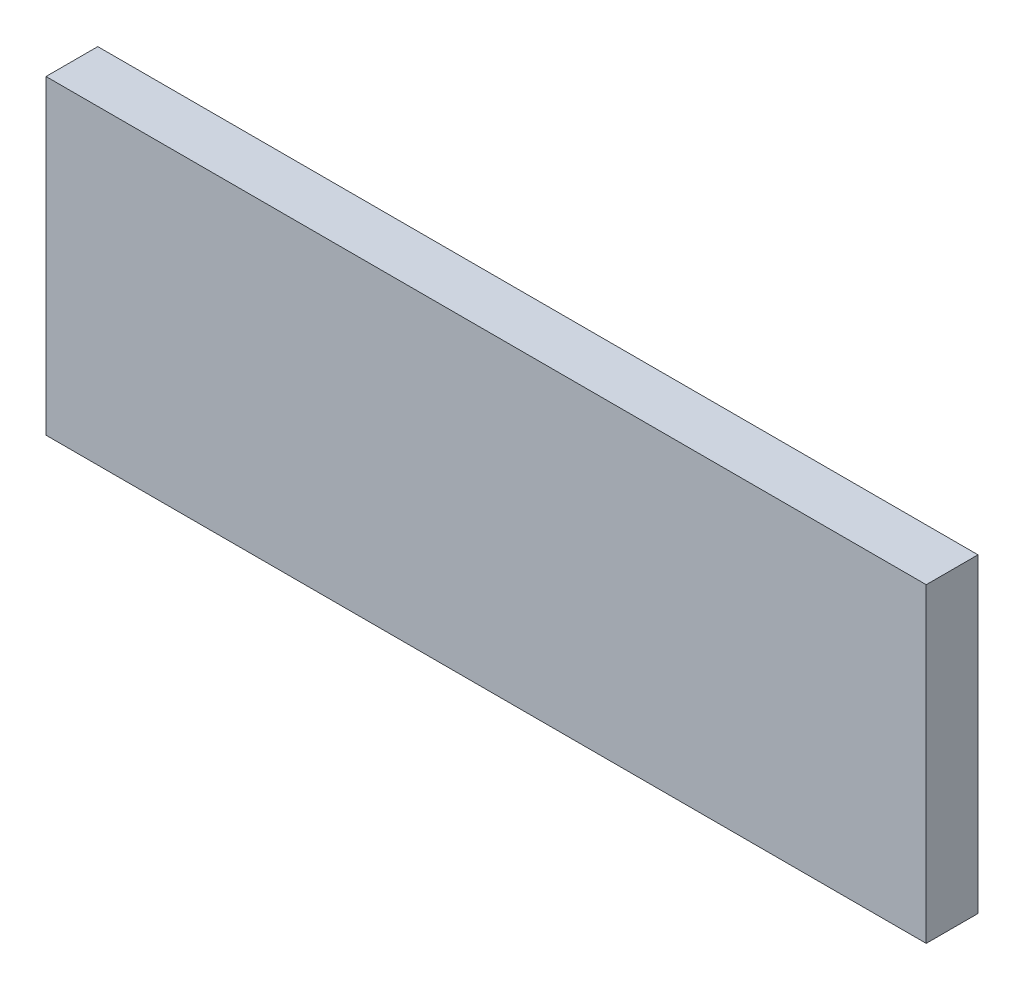
SolidWorks part; units mm, degrees
material "Q235B"
ref_plane "Front Plane" through (0, 0, 0) normal (0, 0, 1) x (1, 0, 0)
ref_plane "Top Plane" through (0, 0, 0) normal (0, 1, 0) x (1, 0, 0)
ref_plane "Right Plane" through (0, 0, 0) normal (1, 0, 0) x (0, 0, -1)
sketch "Sketch1" plane through (0, 0, 0) normal (0, 0, 1) x (1, 0, 0)
  line L1 (0, 0) -> (340, 0)
  line L2 (0, 0) -> (0, 120)
  line L3 (0, 120) -> (340, 120)
  line L4 (340, 0) -> (340, 120)
  dimension "D1" = 340
  dimension "D2" = 120
extrude "Boss-Extrude1" add sketch "Sketch1" along normal blind 20
